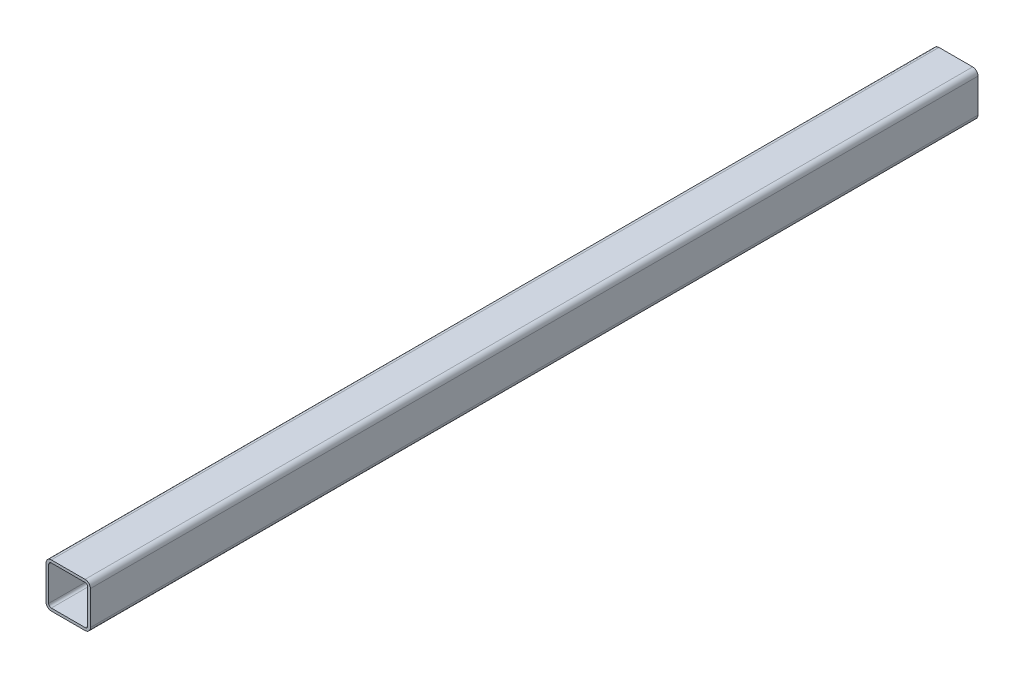
SolidWorks part; units mm, degrees
material "Q235B"
ref_plane "前视基准面" through (0, 0, 0) normal (0, 0, 1) x (1, 0, 0)
ref_plane "上视基准面" through (0, 0, 0) normal (0, 1, 0) x (1, 0, 0)
ref_plane "右视基准面" through (0, 0, 0) normal (1, 0, 0) x (0, 0, -1)
other "Configuration Table"
sketch "草图1" plane through (0, 0, 0) normal (1, 0, 0) x (0, 0, -1)
  line L0 (-500, 0) -> (500, 0)
other "Gb／6728-1986方形空心型钢 050 X 50 X 3(1)"
ref_plane "基准面1" through (0, 0, 500) normal (0, 0, -1) x (0, 1, 0)
sketch "Sketch1" plane through (0, 0, 500) normal (0, 0, -1) x (0, 1, 0)
  line L0 (-19, -22) -> (19, -22)
  line L1 (-22, -19) -> (-22, 19)
  line L2 (19, 22) -> (-19, 22)
  line L3 (22, 19) -> (22, -19)
  line L4 (-19, -25) -> (19, -25)
  line L5 (-25, -19) -> (-25, 19)
  line L6 (19, 25) -> (-19, 25)
  line L7 (25, 19) -> (25, -19)
  arc A0 (25, 19) -> (19, 25) centre (19, 19) ccw
  arc A1 (19, -25) -> (25, -19) centre (19, -19) ccw
  arc A2 (-25, -19) -> (-19, -25) centre (-19, -19) ccw
  arc A3 (-19, 25) -> (-25, 19) centre (-19, 19) ccw
  arc A4 (-19, 22) -> (-22, 19) centre (-19, 19) ccw
  arc A5 (22, 19) -> (19, 22) centre (19, 19) ccw
  arc A6 (19, -22) -> (22, -19) centre (19, -19) ccw
  arc A7 (-22, -19) -> (-19, -22) centre (-19, -19) ccw
  point P0 (-25, 0)
  point P1 (25, 0)
  point P2 (0, 25)
  point P3 (0, -25)
  point P4 (0, 0)
  point P5 (-25, -25)
  point P6 (25, -25)
  point P7 (25, 25)
  point P8 (-25, 25)
  point P33 (0, 0)
  dimension "D1" = 6
  dimension "Thickness" = 3
  dimension "V_leg" = 50
equation "\"D2@草图1\"=\"D1@草图1\"/2"
